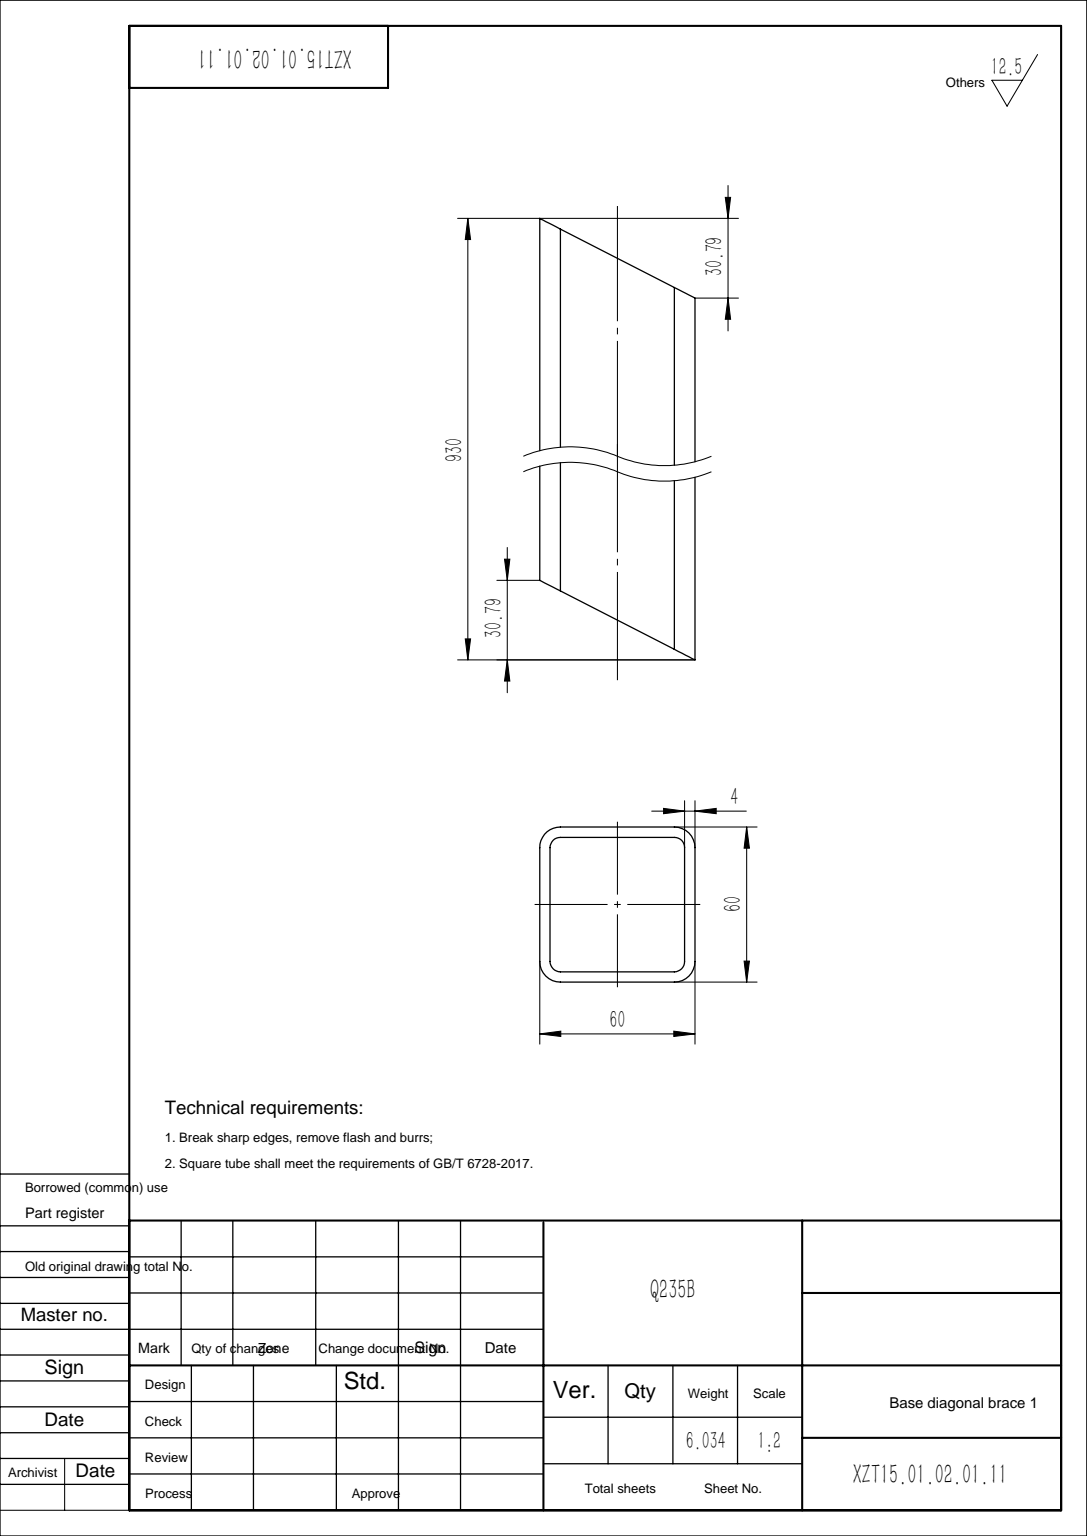
from build123d import *

# Parameters (mm, degrees)
GB_T_6728_2002_SQUARE_HOLLOW_SECTION_60_DEPTH = 930
CUT_EXTRUDE1_DEPTH                            = 933.416216075
CUT_EXTRUDE1_DEPTH_BACK                       = 933.416216075


with BuildPart() as part:
    # Sketch1 → GB/T 6728-2002 square hollow section 60×60×4(1) (new body)
    with BuildSketch(Plane(origin=(0, 0, 0), x_dir=(-1, 0, 0), z_dir=(0, 1, 0))):
        with BuildLine():
            Line((-22, -30), (22, -30))
            ThreePointArc((22, -30), (27.656854249, -27.656854249), (30, -22))
            Line((30, -22), (30, 22))
            ThreePointArc((30, 22), (27.656854249, 27.656854249), (22, 30))
            Line((22, 30), (-22, 30))
            ThreePointArc((-22, 30), (-27.656854249, 27.656854249), (-30, 22))
            Line((-30, 22), (-30, -22))
            ThreePointArc((-30, -22), (-27.656854249, -27.656854249), (-22, -30))
        make_face()
        with BuildLine():
            Line((-22, -26), (22, -26))
            ThreePointArc((22, -26), (24.828427125, -24.828427125), (26, -22))
            Line((26, -22), (26, 22))
            ThreePointArc((26, 22), (24.828427125, 24.828427125), (22, 26))
            Line((22, 26), (-22, 26))
            ThreePointArc((-22, 26), (-24.828427125, 24.828427125), (-26, 22))
            Line((-26, 22), (-26, -22))
            ThreePointArc((-26, -22), (-24.828427125, -24.828427125), (-22, -26))
        make_face(mode=Mode.SUBTRACT)
    extrude(amount=GB_T_6728_2002_SQUARE_HOLLOW_SECTION_60_DEPTH)

    # Sketch2 → Cut-Extrude1 (cut, two sides: drawn at the far end of the back side and taken through both)
    with BuildSketch(Plane.XY.offset(30).offset(-CUT_EXTRUDE1_DEPTH_BACK)):
        Polygon((-30, 930), (30, 899.206782946), (30, 930), align=None)
        Polygon((-30, 0), (-30, 30.793217054), (30, 0), align=None)
    extrude(amount=CUT_EXTRUDE1_DEPTH + CUT_EXTRUDE1_DEPTH_BACK, mode=Mode.SUBTRACT)


solid = part.part
